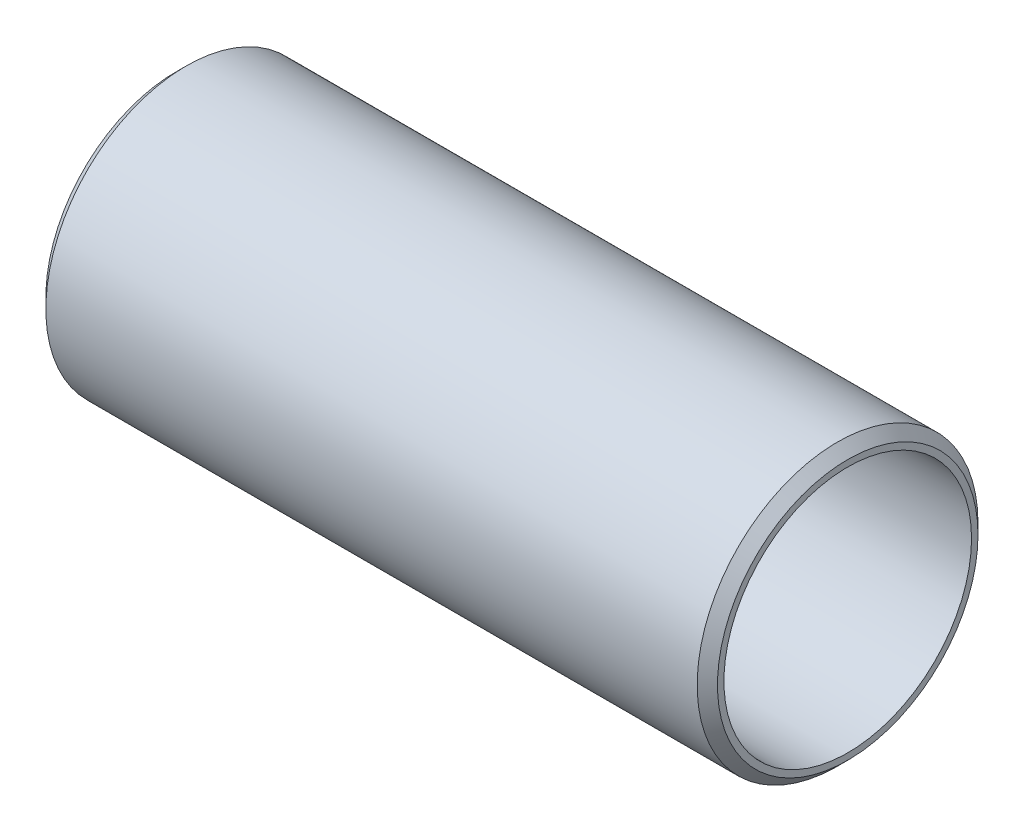
SolidWorks part; units mm, degrees
material "普通碳钢"
ref_plane "前视基准面" through (0, 0, 0) normal (0, 0, 1) x (1, 0, 0)
ref_plane "上视基准面" through (0, 0, 0) normal (0, 1, 0) x (1, 0, 0)
ref_plane "右视基准面" through (0, 0, 0) normal (1, 0, 0) x (0, 0, -1)
sketch "草图1" plane through (0, 0, 0) normal (0, 0, 1) x (1, 0, 0)
  line L0 (0, 0) -> (182, 0)
  dimension "D1" = 182
other "焊接钢管gb∕t3091-2008 Φ76.1X4.5(1)"
ref_plane "基准面1" through (0, 0, 0) normal (1, 0, 0) x (0, 1, 0)
sketch "Sketch1" plane through (0, 0, 0) normal (1, 0, 0) x (0, 1, 0)
  circle A0 centre (0, 0) radius 33.55
  circle A1 centre (0, 0) radius 38.05
  point P3 (0, 0)
  dimension "Out_dia" = 76.1
  dimension "Thickness" = 4.5
chamfer "倒角1" distance 2.75 angle 45 2 edges at (182, 0, -38.05) (0, 0, -38.05)
